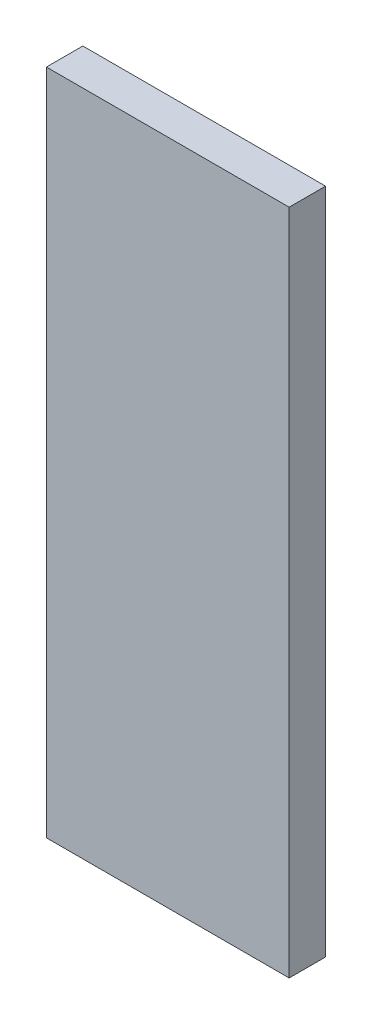
from build123d import *

# Parameters (mm, degrees)
SKETCH1_W           = 40
SKETCH1_H           = 110
BOSS_EXTRUDE1_DEPTH = 6


with BuildPart() as part:
    # Sketch1 → Boss-Extrude1 (new body)
    with BuildSketch(Plane.XY):
        Rectangle(SKETCH1_W, SKETCH1_H)
    extrude(amount=BOSS_EXTRUDE1_DEPTH)


solid = part.part
